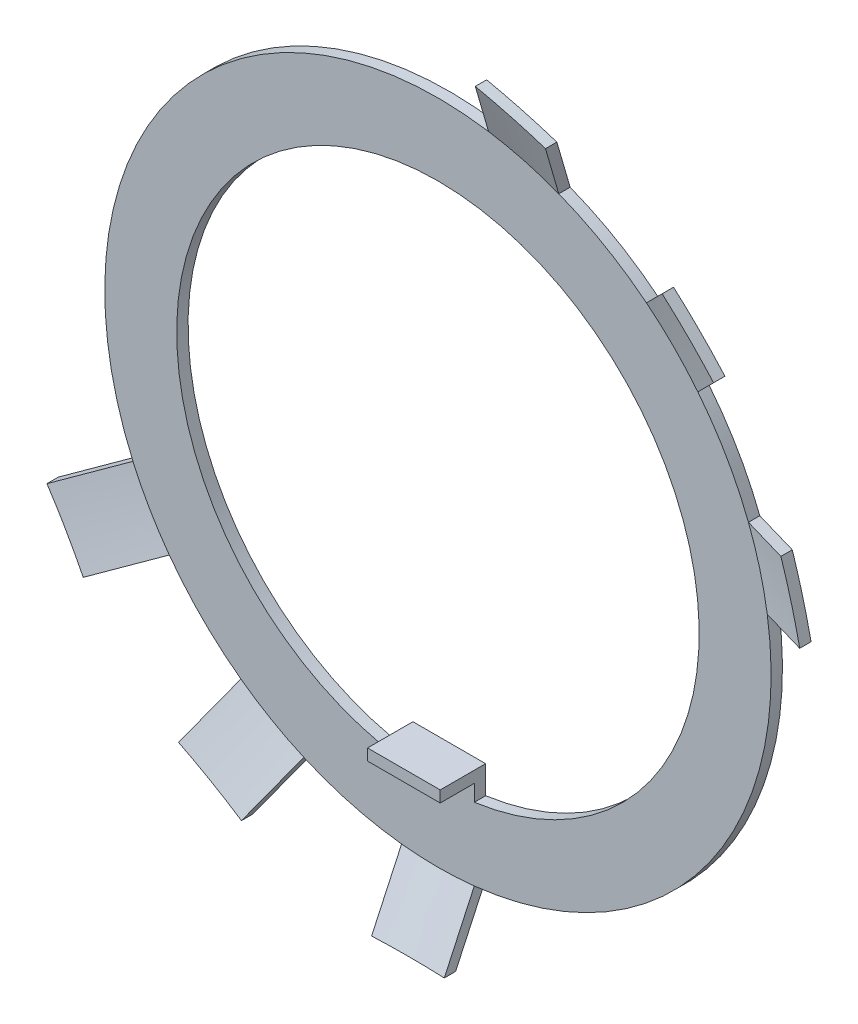
from build123d import *

# Parameters (mm, degrees)
SKETCH3_OUTSIDE_W   = 136.718
SKETCH3_OUTSIDE_H   = 136.718
CUT_EXTRUDE2_DEPTH  = 5.463617
SKETCH4_W           = 9.6
SKETCH4_H           = 1.5
BOSS_EXTRUDE1_DEPTH = 6


with BuildPart() as part:
    # Sketch2 → Base-Revolve (revolve)
    with BuildSketch(Plane(origin=(0, 0, 0), x_dir=(0, 0, -1), z_dir=(1, 0, 0))):
        Polygon((-3.963615094, 52.5), (0, 44), (0, 0), (-1.5, 0), (-1.5, 44), (-5.463615094, 52.5), align=None)
    revolve(axis=Axis((0, 0, 0), (0, 0, 1)))

    # Sketch3 outside → Cut-Extrude2 (cut)
    # profile 1 of 2: a face of its own
    with BuildSketch(Plane.XY):
        Rectangle(SKETCH3_OUTSIDE_W, SKETCH3_OUTSIDE_H)
        with BuildLine():
            Line((-4.8, -43.737398185), (-4.8, -52.280110941))
            Line((-4.8, -52.280110941), (4.8, -52.280110941))
            Line((4.8, -52.280110941), (4.8, -43.737398185))
            ThreePointArc((4.8, -43.737398185), (34.907546973, -26.785502876), (43.489413898, 6.683627667))
            Line((43.489413898, 6.683627667), (51.741040776, 8.894644425))
            Line((51.741040776, 8.894644425), (49.256377943, 18.167532358))
            Line((49.256377943, 18.167532358), (41.004751065, 15.9565156))
            ThreePointArc((41.004751065, 15.9565156), (38.105117767, 22), (34.321123398, 27.532898298))
            Line((34.321123398, 27.532898298), (40.361733517, 33.573508418))
            Line((40.361733517, 33.573508418), (33.573508418, 40.361733517))
            Line((33.573508418, 40.361733517), (27.532898298, 34.321123398))
            ThreePointArc((27.532898298, 34.321123398), (22, 38.105117767), (15.9565156, 41.004751065))
            Line((15.9565156, 41.004751065), (18.167532358, 49.256377943))
            Line((18.167532358, 49.256377943), (8.894644425, 51.741040776))
            Line((8.894644425, 51.741040776), (6.683627667, 43.489413898))
            ThreePointArc((6.683627667, 43.489413898), (-34.907546973, 26.785502876), (-40.277697924, -17.711777154))
            Line((-40.277697924, -17.711777154), (-47.675904188, -21.983133532))
            Line((-47.675904188, -21.983133532), (-42.875904188, -30.296977409))
            Line((-42.875904188, -30.296977409), (-35.477697924, -26.025621031))
            ThreePointArc((-35.477697924, -26.025621031), (-31.112698372, -31.112698372), (-26.025621031, -35.477697924))
            Line((-26.025621031, -35.477697924), (-30.296977409, -42.875904188))
            Line((-30.296977409, -42.875904188), (-21.983133532, -47.675904188))
            Line((-21.983133532, -47.675904188), (-17.711777154, -40.277697924))
            ThreePointArc((-17.711777154, -40.277697924), (-11.388037985, -42.500736357), (-4.8, -43.737398185))
        make_face(mode=Mode.SUBTRACT)
    # profile 2 of 2: a face of its own
    with BuildSketch(Plane.XY):
        with BuildLine():
            Line((4.8, -34.164455213), (4.8, -30.5))
            Line((4.8, -30.5), (-4.8, -30.5))
            Line((-4.8, -30.5), (-4.8, -34.164455213))
            ThreePointArc((-4.8, -34.164455213), (0, 34.5), (4.8, -34.164455213))
        make_face()
    extrude(amount=CUT_EXTRUDE2_DEPTH, mode=Mode.SUBTRACT)

    # Sketch4 → Boss-Extrude1 (add)
    with BuildSketch(Plane.XY):
        with Locations((0, -31.25)):
            Rectangle(SKETCH4_W, SKETCH4_H)
    extrude(amount=BOSS_EXTRUDE1_DEPTH)


solid = part.part
